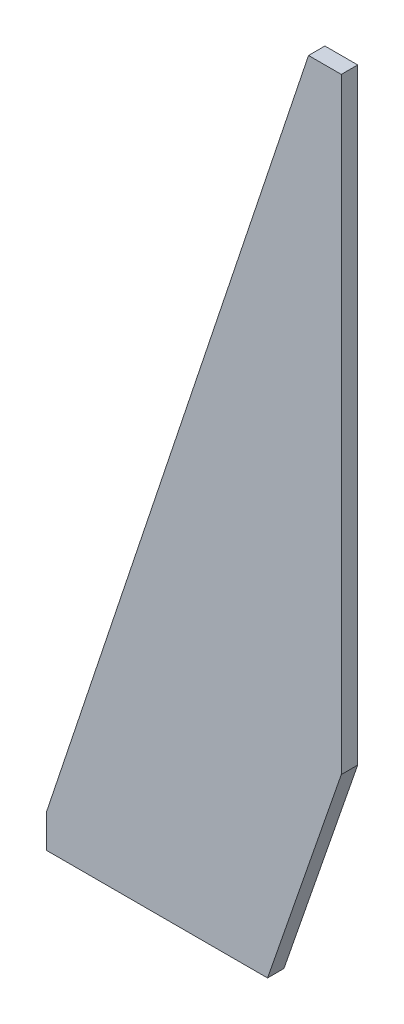
SolidWorks part; units mm, degrees
material "普通碳钢"
ref_plane "Front Plane" through (0, 0, 0) normal (0, 0, 1) x (1, 0, 0)
ref_plane "Top Plane" through (0, 0, 0) normal (0, 1, 0) x (1, 0, 0)
ref_plane "Right Plane" through (0, 0, 0) normal (1, 0, 0) x (0, 0, -1)
sketch "Sketch1" plane through (0, 0, 0) normal (0, 0, 1) x (1, 0, 0)
  line L0 (0, 130) -> (0, 500)
  line L1 (0, 500) -> (-20, 500)
  line L2 (-20, 500) -> (-180, 20)
  line L3 (-180, 20) -> (-180, 0)
  line L4 (-180, 0) -> (-45, 0)
  line L5 (-45, 0) -> (0, 130)
  dimension "D1" = 500
  dimension "D2" = 130
  dimension "D3" = 20
  dimension "D4" = 20
  dimension "D5" = 180
  dimension "D6" = 45
extrude "Boss-Extrude1" add sketch "Sketch1" along normal mid plane 10
